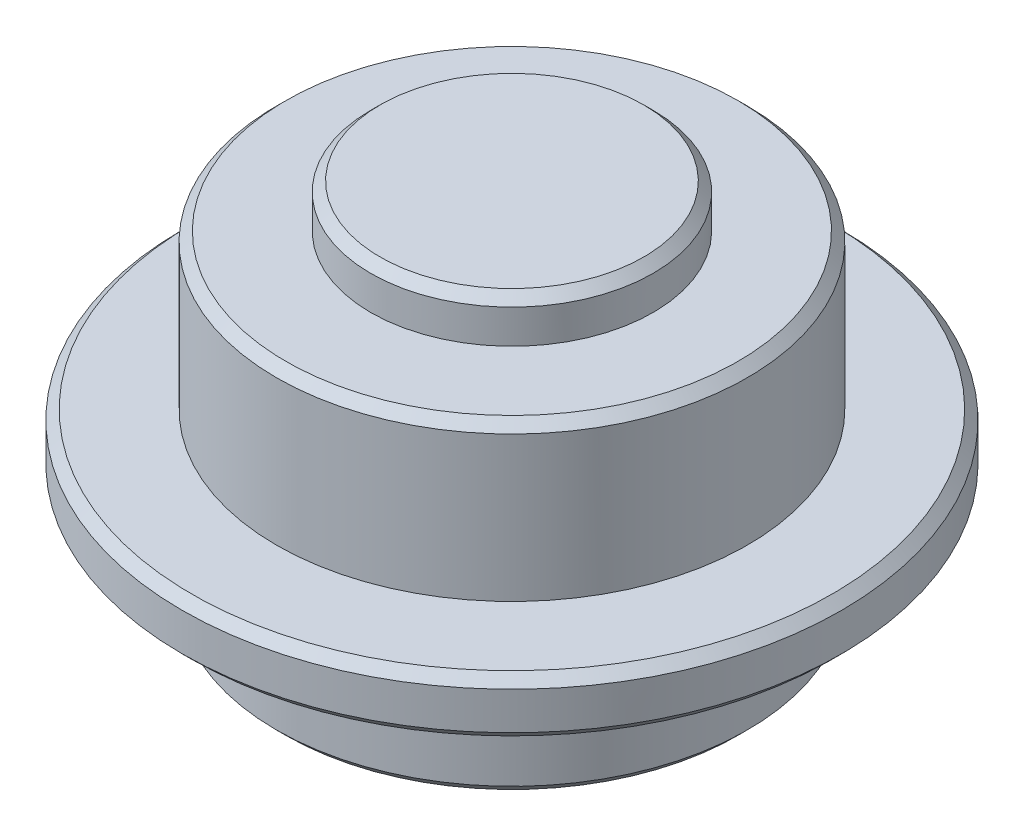
SolidWorks part; units mm, degrees
material "Q235B"
ref_plane "Front Plane" through (0, 0, 0) normal (0, 0, 1) x (1, 0, 0)
ref_plane "Top Plane" through (0, 0, 0) normal (0, 1, 0) x (1, 0, 0)
ref_plane "Right Plane" through (0, 0, 0) normal (1, 0, 0) x (0, 0, -1)
sketch "Sketch1" plane through (0, 0, 0) normal (0, 0, 1) x (1, 0, 0)
  line L0 (380.5, -9.2) -> (380.5, -3.2)
  line L1 (380.5, -3.2) -> (385.5, -3.2)
  line L2 (385.5, -3.2) -> (385.5, -0.2)
  line L3 (385.5, -0.2) -> (380.5, -0.2)
  line L4 (375.5, 8) -> (375.5, 10.3)
  line L6 (368, 10.3) -> (368, -9.2) construction
  line L7 (384.2, 10.3) -> (351.8, 10.3) construction
  line L8 (-425, -9.2) -> (425, -9.2) construction
  line L9 (380.5, -9.2) -> (368, -9.2)
  line L10 (375.5, 10.3) -> (368, 10.3)
  line L11 (368, 10.3) -> (368, -9.2)
  line L12 (380.5, -0.2) -> (380.5, 8)
  line L13 (384.2, 8) -> (351.8, 8) construction
  line L14 (380.5, 8) -> (375.5, 8)
  dimension "D1" = 3
revolve "Revolve1" add sketch "Sketch1" angle 360 about L6
chamfer "Chamfer1" distance 0.5 angle 45 5 edges at (368, -9.2, 12.5) (368, -3.2, 17.5) (368, -0.2, 17.5) (368, 8, 12.5) (368, 10.3, 7.5)
